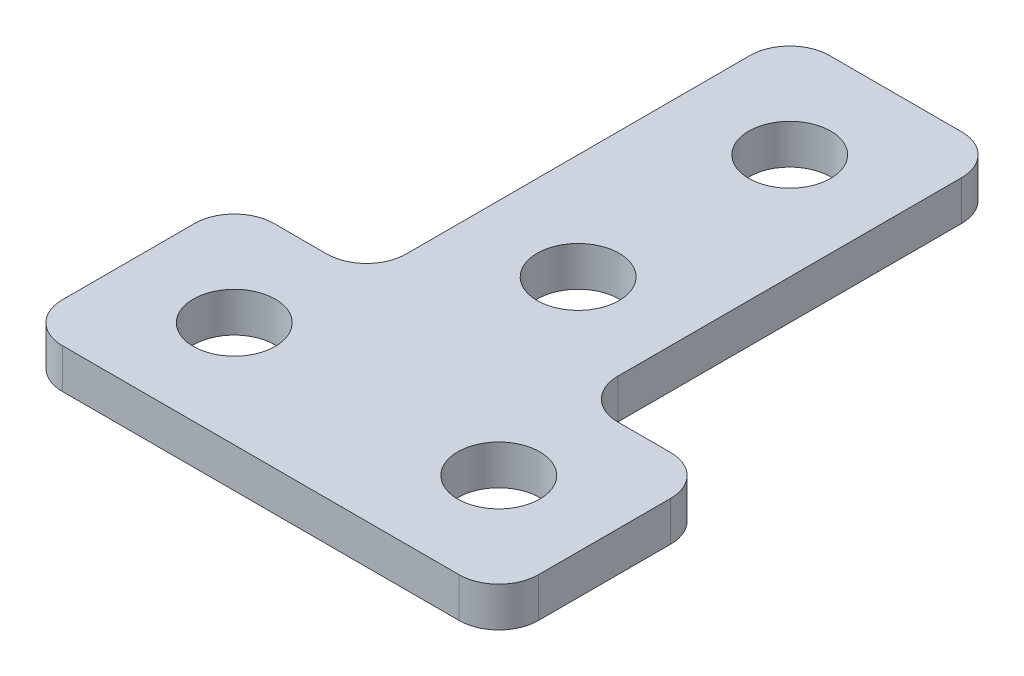
from build123d import *

# Parameters (mm, degrees)
SKETCH_1_R      = 1.55
EXTRUDE_1_DEPTH = 1.5
FILLET_1_R      = 1.5


with BuildPart() as part:
    # 草图1 → 凸台-拉伸1 (new body)
    with BuildSketch(Plane(origin=(0, 0, 0), x_dir=(1, 0, 0), z_dir=(0, 1, 0))):
        Polygon((-4, 20), (4, 20), (4, 4), (9, 4), (9, -4), (-9, -4), (-9, 4), (-4, 4), align=None)
        with Locations(Location((5, 0, 0), (0, 0, 270))):
            Circle(SKETCH_1_R, mode=Mode.SUBTRACT)
        with Locations(Location((0, 8, 0), (0, 0, 270))):
            Circle(SKETCH_1_R, mode=Mode.SUBTRACT)
        with Locations(Location((0, 16, 0), (0, 0, 270))):
            Circle(SKETCH_1_R, mode=Mode.SUBTRACT)
        with Locations(Location((-5, 0, 0), (0, 0, 90))):
            Circle(SKETCH_1_R, mode=Mode.SUBTRACT)
    extrude(amount=EXTRUDE_1_DEPTH)

    # 圆角1
    fillet_1_edges = [part.edges().sort_by_distance(p)[0] for p in [
        (4, 0.75, -4),
        (9, 0.75, -4),
        (9, 0.75, 4),
        (-9, 0.75, 4),
        (-9, 0.75, -4),
        (-4, 0.75, -4),
        (-4, 0.75, -20),
        (4, 0.75, -20),
    ]]
    fillet(fillet_1_edges, radius=FILLET_1_R)


solid = part.part
